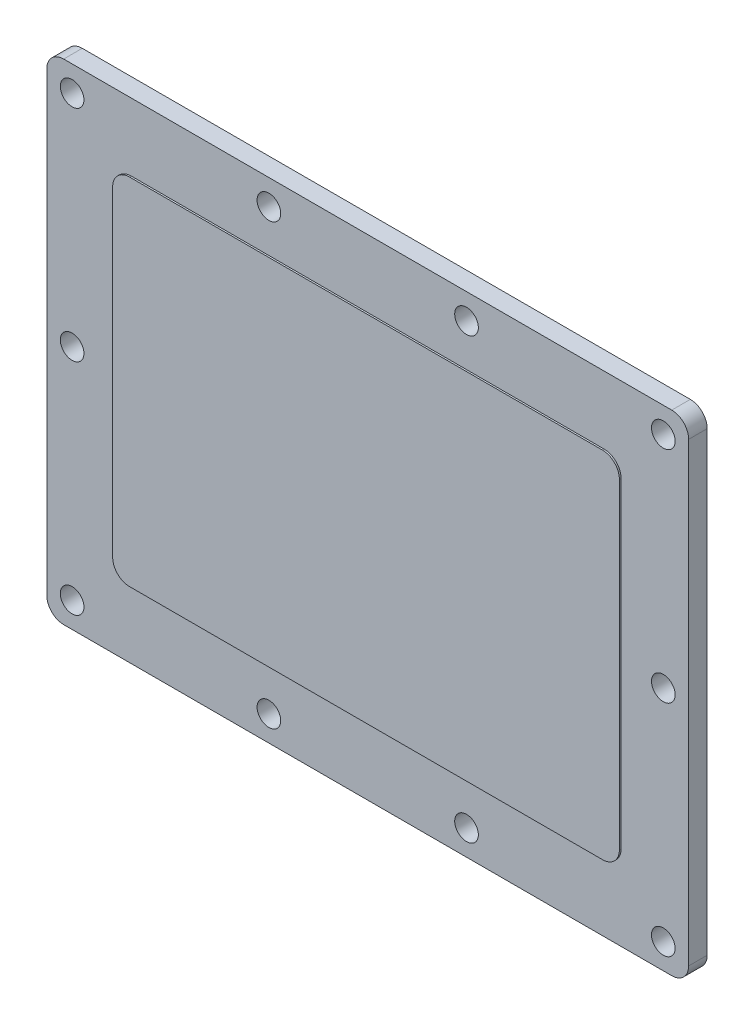
SolidWorks part; units mm, degrees
material "Q235"
ref_plane "Front Plane" through (0, 0, 0) normal (0, 0, 1) x (1, 0, 0)
ref_plane "Top Plane" through (0, 0, 0) normal (0, 1, 0) x (1, 0, 0)
ref_plane "Right Plane" through (0, 0, 0) normal (1, 0, 0) x (0, 0, -1)
sketch "Sketch1" plane through (0, 0, 0) normal (0, 0, 1) x (1, 0, 0)
  line L1 (10, 0) -> (370, 0)
  line L2 (0, 10) -> (0, 280)
  line L3 (10, 290) -> (370, 290)
  line L4 (380, 10) -> (380, 280)
  arc A1 (10, 0) -> (0, 10) centre (10, 10) cw
  arc A2 (370, 0) -> (380, 10) centre (370, 10) ccw
  arc A5 (370, 290) -> (380, 280) centre (370, 280) cw
  arc A7 (0, 280) -> (10, 290) centre (10, 280) cw
  circle A8 centre (15, 275) radius 7
  circle A9 centre (131.5, 275) radius 7
  circle A10 centre (248.5, 275) radius 7
  circle A11 centre (365, 275) radius 7
  circle A12 centre (365, 145) radius 7
  circle A13 centre (365, 15) radius 7
  circle A14 centre (248.5, 15) radius 7
  circle A15 centre (131.5, 15) radius 7
  circle A16 centre (15, 15) radius 7
  circle A17 centre (15, 145) radius 7
  point P14 (0, 0)
  point P17 (380, 0)
  point P30 (0, 290)
  dimension "D7" = 260
  dimension "D3" = 14
  dimension "D4" = 350
  dimension "D5" = 15
  dimension "D6" = 15
  dimension "D8" = 117
  dimension "D9" = 130
  dimension "D10" = 116.5
  dimension "D1" = 380
  dimension "D2" = 290
extrude "Boss-Extrude1" add sketch "Sketch1" along normal blind 12
sketch "Sketch2" plane through (0, 0, 12) normal (0, 0, 1) x (1, 0, 0)
  line L0 (10, 0) -> (370, 0) construction
  line L1 (50, 250) -> (330, 250)
  line L2 (40, 240) -> (40, 50)
  line L3 (50, 40) -> (330, 40)
  line L4 (340, 240) -> (340, 50)
  line L5 (0, 280) -> (0, 10) construction
  arc A0 (330, 250) -> (340, 240) centre (330, 240) cw
  arc A1 (330, 40) -> (340, 50) centre (330, 50) ccw
  arc A2 (40, 50) -> (50, 40) centre (50, 50) ccw
  arc A3 (50, 250) -> (40, 240) centre (50, 240) ccw
  point P12 (340, 40)
  point P15 (40, 40)
  point P18 (40, 250)
  dimension "D5" = 10
  dimension "D1" = 300
  dimension "D2" = 210
  dimension "D3" = 40
  dimension "D4" = 40
extrude "Cut-Extrude1" cut sketch "Sketch2" against normal blind 1 flip side to cut
